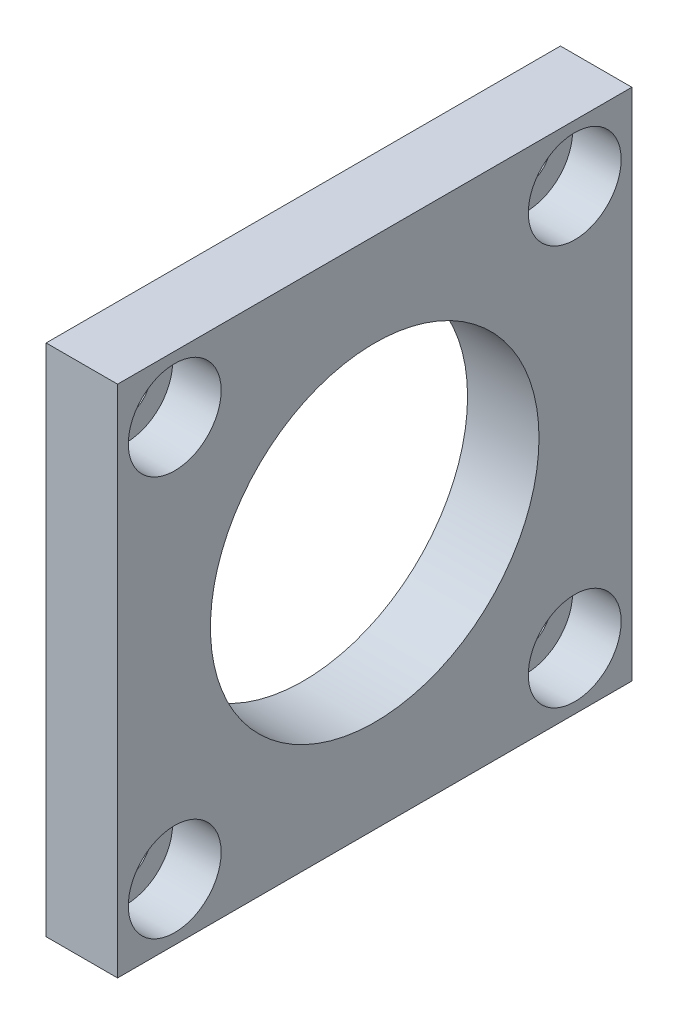
from build123d import *

# Parameters (mm, degrees)
SKETCH1_W                                           = 36
SKETCH1_H                                           = 36
BOSS_EXTRUDE1_DEPTH                                 = 2.5
CBORE_FOR_M3_HEX_SOCKET_HEAD_CAP_SCREW1_D           = 3.4
CBORE_FOR_M3_HEX_SOCKET_HEAD_CAP_SCREW1_CBORE_D     = 6.5
CBORE_FOR_M3_HEX_SOCKET_HEAD_CAP_SCREW1_CBORE_DEPTH = 3.4
SKETCH5_R                                           = 11.5
CUT_EXTRUDE2_DEPTH                                  = 26.942243542


with BuildPart() as part:
    # Sketch1 → Boss-Extrude1 (new, symmetric)
    with BuildSketch(Plane(origin=(0, 0, 0), x_dir=(0, 0, -1), z_dir=(1, 0, 0))):
        Rectangle(SKETCH1_W, SKETCH1_H)
    extrude(amount=BOSS_EXTRUDE1_DEPTH, both=True)

    # CBORE for M3 Hex Socket Head Cap Screw1 (through all)
    with Locations(Plane(origin=(2.5, 0, 0), x_dir=(0, 0, -1), z_dir=(1, 0, 0))):
        with Locations((-14, 14), (14, 14), (-14, -14), (14, -14)):
            CounterBoreHole(CBORE_FOR_M3_HEX_SOCKET_HEAD_CAP_SCREW1_D / 2, CBORE_FOR_M3_HEX_SOCKET_HEAD_CAP_SCREW1_CBORE_D / 2, CBORE_FOR_M3_HEX_SOCKET_HEAD_CAP_SCREW1_CBORE_DEPTH)

    # Sketch5 → Cut-Extrude2 (cut, through all)
    with BuildSketch(Plane(origin=(2.5, 0, 0), x_dir=(0, 0, -1), z_dir=(1, 0, 0))):
        Circle(SKETCH5_R)
    extrude(amount=-CUT_EXTRUDE2_DEPTH, mode=Mode.SUBTRACT)


solid = part.part
